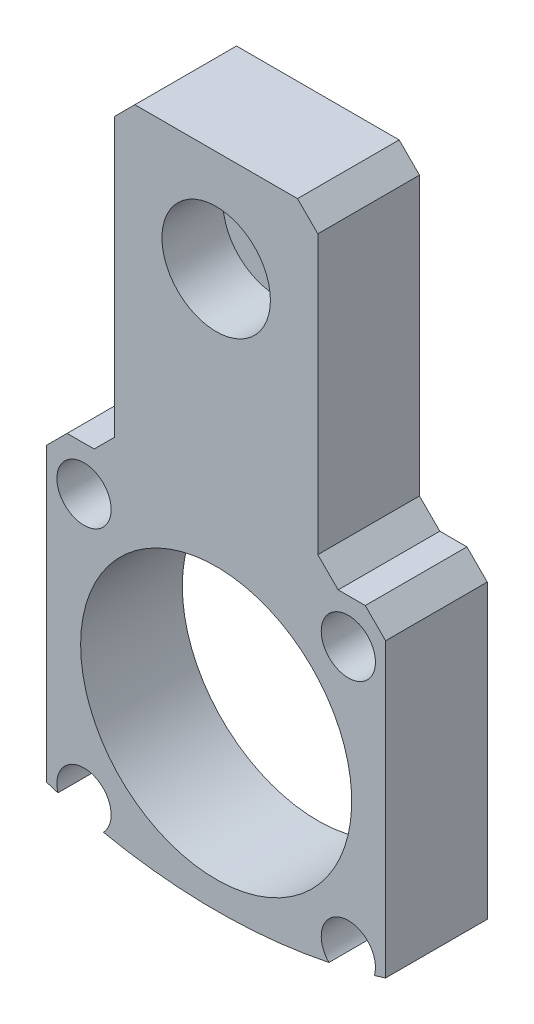
from build123d import *

# Parameters (mm, degrees)
SKETCH1_W           = 50
SKETCH1_H           = 97
BOSS_EXTRUDE1_DEPTH = 15
SKETCH6_R           = 8
CUT_EXTRUDE3_DEPTH  = 9
SKETCH7_R           = 4.5
CUT_EXTRUDE4_DEPTH  = 57.444472183
SKETCH8_R           = 20
SKETCH8_R_2         = 4
CUT_EXTRUDE5_DEPTH  = 58.705965376
SKETCH9_W           = 32.009633737
SKETCH9_H           = 62.03619176
SKETCH9_W_2         = 30.458131691
SKETCH9_H_2         = 52.571237354
CUT_EXTRUDE6_DEPTH  = 58.705965376
CHAMFER1_SIZE       = 3
SKETCH14_R          = 119.720313389
SKETCH14_R_2        = 82
CUT_EXTRUDE10_DEPTH = 58.705965376


with BuildPart() as part:
    # Sketch1 → Boss-Extrude1 (new body)
    with BuildSketch(Plane.XY):
        with Locations((-0.2255048, 1.185534591)):
            Rectangle(SKETCH1_W, SKETCH1_H)
    extrude(amount=BOSS_EXTRUDE1_DEPTH)

    # Sketch6 → Cut-Extrude3 (cut)
    with BuildSketch(Plane.XY.offset(15)):
        with Locations((-0.2255048, 34.685534591)):
            Circle(SKETCH6_R)
    extrude(amount=-CUT_EXTRUDE3_DEPTH, mode=Mode.SUBTRACT)

    # Sketch7 → Cut-Extrude4 (cut, through all)
    with BuildSketch(Plane.XY.offset(6)):
        with Locations((-0.2255048, 34.685534591)):
            Circle(SKETCH7_R)
    extrude(amount=-CUT_EXTRUDE4_DEPTH, mode=Mode.SUBTRACT)

    # Sketch8 → Cut-Extrude5 (cut, through all)
    with BuildSketch(Plane(origin=(0, 0, 0), x_dir=(-1, 0, 0), z_dir=(0, 0, -1))):
        with Locations((0.2255048, -23.314465409)):
            Circle(SKETCH8_R)
        with Locations((-19.2744952, -42.814465409)):
            Circle(SKETCH8_R_2)
        with Locations((-19.2744952, -3.814465409)):
            Circle(SKETCH8_R_2)
        with Locations((19.7255048, -3.814465409)):
            Circle(SKETCH8_R_2)
        with Locations((19.7255048, -42.814465409)):
            Circle(SKETCH8_R_2)
    extrude(amount=-CUT_EXTRUDE5_DEPTH, mode=Mode.SUBTRACT)

    # Sketch9 → Cut-Extrude6 (cut, through all)
    with BuildSketch(Plane.XY.offset(15)):
        with Locations((30.779312069, 33.703630471)):
            Rectangle(SKETCH9_W, SKETCH9_H)
        with Locations((-30.454570646, 28.971153268)):
            Rectangle(SKETCH9_W_2, SKETCH9_H_2)
    extrude(amount=-CUT_EXTRUDE6_DEPTH, mode=Mode.SUBTRACT)

    # Chamfer1
    chamfer1_edges = [part.edges().sort_by_distance(p)[0] for p in [
        (14.7744952, 49.685534591, 7.5),
        (14.7744952, 2.685534591, 7.5),
        (24.7744952, 2.685534591, 7.5),
        (-15.2255048, 49.685534591, 7.5),
        (-25.2255048, 2.685534591, 7.5),
        (-15.2255048, 2.685534591, 7.5),
    ]]
    chamfer(chamfer1_edges, length=CHAMFER1_SIZE)

    # Sketch14 → Cut-Extrude10 (cut, through all)
    with BuildSketch(Plane(origin=(0, 0, 0), x_dir=(-1, 0, 0), z_dir=(0, 0, -1))):
        with Locations((0.2255048, 34.685534591)):
            Circle(SKETCH14_R)
        with Locations((0.2255048, 34.685534591)):
            Circle(SKETCH14_R_2, mode=Mode.SUBTRACT)
    extrude(amount=-CUT_EXTRUDE10_DEPTH, mode=Mode.SUBTRACT)


solid = part.part
